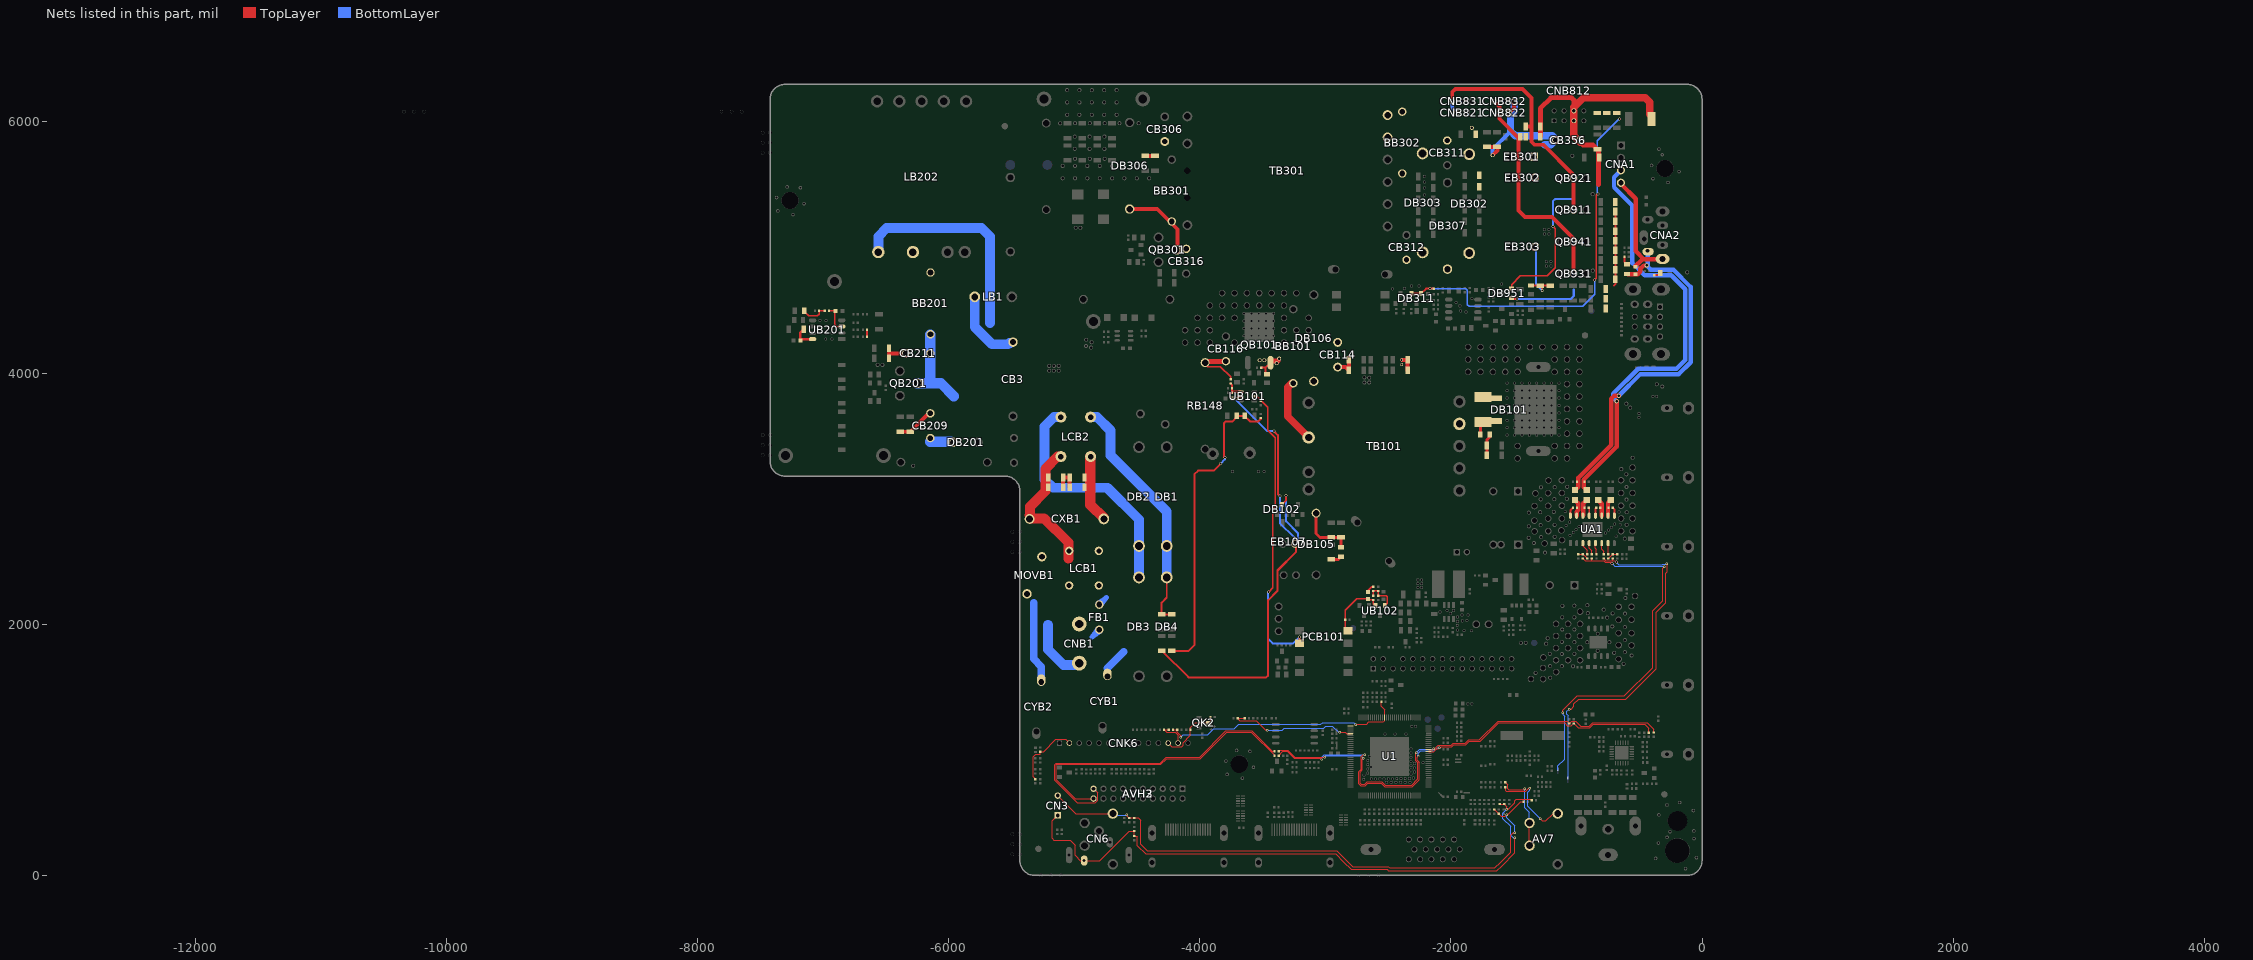
[diagram p0: the nets of this part, all layers, seen from the top]
# Altium PCB MISC84277.PcbDoc (part 11 of 15)
Units mil, origin at the board's own origin, x right, y up, seen from the top; angles counter-clockwise.
Board outline 7422.08 x 6299.21 mil, 2 copper layers (TopLayer, BottomLayer), stack 61.855 mil thick; 709 components, 395 nets, 2812 pads, 811 vias.

## Via types
v1: diameter 23.62, hole 15.75, TopLayer to BottomLayer, tented both sides, 437 vias
v2: diameter 19.68, hole 11.81, TopLayer to BottomLayer, tented both sides, 353 vias
v3: diameter 31.5, hole 23.62, TopLayer to BottomLayer, tented both sides, 16 vias
v4: diameter 31.5, hole 19.68, TopLayer to BottomLayer, tented both sides, 4 vias
v5: diameter 17.72, hole 9.84, TopLayer to BottomLayer, tented both sides, 1 vias

## Nets (pads, with @x,y where several pads share a name; then routed paths per layer and width w, separated by ;. In a path a pad name is that pad's centre, name@x,y a point inside that pad or via, vN(x,y) a via of type N, cw(c..) or ccw(c..) an arc to the next point about the centre after c; other vN are vias at no path point) (continued)
K7: CNK6.2 RK5.2 RK6.2 | length 552.8
  TopLayer w5: RK6.2@-5308.96,769.93 -5312.43,769.93 -5327.79,785.29 -5327.79,943.38 -5308.61,962.56 -5274.6,962.56 -5271.45,965.71 RK5.2@-5271.45,984.62 -5244.79,984.62 -5146.96,1082.45 -5068.22,1082.45 CNK6.2@-5039.07,1053.3
KEY: CK2.1 RK3.1 U1.101 | length 1020.6
  TopLayer w6: RK3.1@-3642.73,1251 CK2.1@-3698.27,1250.99 -3680.43,1233.16 -3551.66,1233.16 -3475.5,1157 v2@-3464.3,1157 ; v2@-2883,1139 -2842.97,1139 -2831.75,1127.78 U1.101@-2800.46,1127.78
  BottomLayer w6: v2@-3464.3,1157 -3344.2,1157 -3328.78,1172.42 -3012.14,1172.42 -2995.56,1189 -2944.68,1189 v2@-2893.68,1138
  other v2: -2884,1138 -3462.8,1156.4
L: DB1.A DB4.K LCB2.3 RB101.1 RB141.2 | length 1949.2
  TopLayer w15.75: DB4.K@-4263.49,2373.12 -4263.49,2213.01 -4304.29,2172.21 RB101.1@-4304.29,2078.76 RB141.2@-4224.49,2078.76
  BottomLayer w78.74: LCB2.3@-4869.89,3650.02 -4818.62,3650.02 -4710,3541.4 -4710,3344.3 -4263.49,2897.79 DB4.K@-4263.49,2373.12
L-1: CNB1.1 FB1.1
L-2: FB1.2 LCB1.2@-4804.49,2308.7
L-3: CXB1.1 CYB1.2 LCB1.3@-4804.49,2584.3 LCB2.2 MOVB1.2@-5258.54,2537.24 RB1.1 RB2.1 | length 723.5
  TopLayer w82.68: LCB2.2@-4869.89,3335.06 -4872.2,3332.74 -4872.2,2952.78 CXB1.1@-4762.92,2843.5
  BottomLayer w59.06: -4735.81,1650.69 -4604.51,1781.99
L-N: RB1.2 RB2.2 RB3.1 RB4.1 | length 209
  TopLayer w31.5: RB4.1@-5089.33,3090.94 RB3.1@-5089.33,3169.17 RB1.2@-5036.74,3169.17 RB2.2@-5036.74,3090.94
LED1: CNB821.2 CNB831.3 DB951.3 QB911.C QB921.C RB905.1 | length 3165.6
  TopLayer w11.81: DB951.3@-1517.68,4674.29 -1517.68,4705.32 -1447.41,4775.59 -1234.25,4775.59 -1171.26,4838.58 -1171.26,5150.26 v1(-1189,5168)
  TopLayer w31.5: CNB831.3@-1989.88,6163.14 -1989.88,6237.58 -1964.5,6262.96 -1431.77,6262.96 -1358.2,6189.4 -1358.2,5968.4 ; RB905.1@-1392,5963.8 -1362.8,5963.8 -1358.2,5968.4 ; QB911.C@-1022.5,5307.26 -1022.5,5578 -1263,5818.5 -1334.2,5818.5 -1358.2,5842.5 -1358.2,5968.4
  BottomLayer w15.75: v1(-1189,5168) -1189,5367.5 -1170,5386.5 -1039.5,5386.5 -1022.5,5369.5 QB911.C@-1022.5,5307.26
  BottomLayer w31.5: CNB831.3@-1989.88,6163.14 -1989.88,6111.52 CNB821.2@-1950.51,6072.15
LED2: CNB822.2 CNB832.3 DB951.1 JB102.2 JB107.1 pad.VIA5@-1833.15,5953.3 QB931.C QB941.C RB904.1 | length 2353.7
  TopLayer w19.68: DB951.1@-1517.68,4599.29 -1508.89,4590.5 v1(-1475,4590.5)
  TopLayer w31.5: CNB832.3@-1654.61,6163.14 -1615.24,6123.77 CNB822.2@-1615.24,6072.15 -1615.24,6026.66 -1469.78,5881.2 -1445.6,5881.2 -1460.63,5866.17 -1460.63,5295.28 -1409.45,5244.09 -1194.96,5244.09 -1022.5,5071.63 QB931.C@-1022.5,4792.7
  BottomLayer w19.68: v1@-1475,4590.13 -1350,4590.13 ; -1362,4590.13 -1350,4590.13 ; -1022.5,4662.5 -1022.5,4614 -1046.37,4590.13 -1350,4590.13
LED+: CB312.2 CB356.2 CNB822.1 CNB832.1 DB302.K DB303.K DB307.A EB301.1 EB302.1 EB303.1 JB103.1 JB106.1 pad.VIA5@-1668.9,5735.1 RB358.1 RB360.2 RB363.2 | length 1818.8
  TopLayer w15.75: RB358.1@-1363,4697.59 RB363.2@-1210.69,4697.59 ; RB360.2@-1288.48,4696.65 -1274.94,4696.65 -1273,4694.71 v1(-1273,4658)
  TopLayer w31.5: JB103.1@-1714.4,5801.14 -1714,5801.54 JB106.1@-1632.9,5801.54 ; pad.VIA5@-1668.9,5735.1 -1630.5,5773.5 -1630.5,5800.44 JB106.1@-1616.88,5800.44 ; CNB822.1@-1536.5,6072.15 -1497.13,6111.52 CNB832.1@-1497.13,6163.14
  BottomLayer w15.75: EB303.1@-1322.83,4988.76 -1322.83,4707.83 v1(-1273,4658)
  BottomLayer w31.5: pad.VIA5@-1669.2,5735.1 -1669.2,5782.9 -1539.5,5912.6 ; -1298.2,5889.5 -1297.2,5890.5
  BottomLayer w59.06: CNB832.1@-1497.13,6163.14 -1497.13,6085.87 -1526,6057 -1526,5927.7 -1487.8,5889.5 -1298.2,5889.5 -1192.43,5889.5 -1163.28,5860.35 CB356.2@-1167.43,5856.2 -1205.63,5818 -1253.36,5818
LED_FB: CB356.1 CNB812.5 CNB812.6 DB310.A DB311.1 DB311.3 RB337.2 RB338.2 RB339.2 RB340.2 RB341.2 RB351.1 RB904.2 RB905.2 RB911.1 RB912.1 RB913.1 RB921.1 RB922.1 RB923.1 RB931.1 RB932.1 RB933.1 RB941.1 RB942.1 RB943.1 | length 5802.8
  TopLayer w11.81: v1(-856.3,4740.15) -842.39,4754.05 -842.39,5415.21 v1(-830.7,5426.9)
  TopLayer w15.75: DB311.3@-2312.5,4634.5 DB311.1@-2237.5,4634.5 -2198.57,4673.43 v1@-2168.5,4673.43 ; v1@-2165.5,4673.43 RB351.1@-2137.3,4673.43 ; -702.13,4696.87 -690.23,4708.77 RB922.1@-690.23,5274
  TopLayer w39.37: RB904.2@-1287.5,5888.74 -1287.5,6108.49 -1202.49,6193.5 -1041.02,6193.5 -1020.8,6173.28 -1020.8,6117.2 CNB812.6@-1020.8,6088.35 ; CB356.1@-970.07,5838.83 -949.25,5818 -870.5,5818 -824.5,5772 -824.5,5502.9
  TopLayer w59.06: CNB812.6@-1020.8,6088.35 CNB812.5@-1020.8,6009.61 -1020.8,5889.55 CB356.1@-970.07,5838.83 ; -1020.8,6117.2 -944.5,6193.5 -453.3,6193.5 -418,6158.2 DB310.A@-418,6061.2
  BottomLayer w11.81: v1(-2168.5,4672) -1883,4672 -1869,4658 -1869,4545.63 -1856,4532.63 -950.16,4532.63 -856.3,4626.49 v1(-856.3,4740.15) ; v1(-830.7,5426.9) -834.65,5430.85 -834.65,5849.75 v1(-659,6025.4)
LED_G: CK3.2 CNK6.12 QK2.C RK2.1 | length 504.6
  TopLayer w5: CNK6.12@-4251.67,1053.3 -4222.07,1023.7 -4143.8,1023.7 -4132.9,1034.6 -4132.9,1055.82 -4074.87,1113.85 CK3.2@-4074.87,1160.01 CK3.2@-4074.87,1160.6 ; CK3.2@-4075.16,1160.3 CK3.2@-4074.87,1160.6 ; QK2.C@-3940.33,1213.8 -4036.04,1213.8 -4074.87,1174.97 CK3.2@-4074.87,1160.6 ; QK2.C@-3929.37,1213.8 -3914.23,1228.94 RK2.1@-3914.23,1261.1
LED_R: CK10.2 CNK6.13 RK21.2 | length 229.8
  TopLayer w6: RK21.2@-4247.33,1160 -4284.46,1160 -4263.86,1139.4 -4195.9,1139.4 -4172.93,1116.43 CNK6.13@-4172.93,1053.3
LED_RED: RK18.1 RK20.2 RK21.1 U1.83 | length 1989.4
  TopLayer w6: RK21.1@-4213.87,1160 RK20.2@-4179.33,1160 -4179.33,1138.39 -4152.1,1111.16 v2(-4152.1,1100.4) ; v2(-2759,1200) -2756.5,1202.5 -2671.94,1202.5 -2652.94,1221.5 -2537.5,1221.5 -2528.81,1230.19 U1.83@-2528.81,1257.7 -2528.81,1320.37 -2553.73,1345.29 RK18.1@-2553.73,1381
  BottomLayer w6: v2(-4152.1,1100.4) -4131.83,1120.67 -4033.4,1120.67 ; -4062.3,1120.67 -4033.4,1120.67 ; v2@-2761,1198 v2(-2759,1200) -2776,1217 -3022.8,1217 -3037.8,1202 -3691.04,1202 -3725.69,1167.36 -3888.63,1167.36 -3935.32,1120.67 -4033.4,1120.67
LINEOUT-L: CN3.3 CN6.3 CO4.1 CO10.2 R2.2 RO7.2 RO15.2 | length 4702.3
  TopLayer w6: CN3.3@-5131.53,624.33 CN3.3@-5131.53,635.1 -4988.41,491.97 CN6.3@-4688.98,491.97 ; -2852.12,141.88 -2780.29,70.06 -2499.27,70.06 -2488.59,59.38 -1649.74,59.38 -1604.62,104.5
  TopLayer w8: v2(-4581.5,483.9) -4581.5,474.88 RO7.2@-4563.06,456.43 ; RO7.2@-4563.06,457.03 -4488.93,457.03 -4470.5,438.6 -4470.5,409.5 ; -4470.5,433.5 -4470.5,409.5 ; -2852.12,141.88 -2907.73,197.5 -4420.45,197.5 -4470.5,247.55 -4470.5,409.5 ; RO15.2@-1655,523.73 -1651.46,523.73 CO4.1@-1618,490.27 -1618,489 -1599,470 -1567,470 -1559.32,477.68 -1559.32,479.68 -1555.32,479.68 v2(-1555.32,483.07) -1547.05,483.07 -1445.85,584.27 -1422.73,584.27 R2.2@-1422.73,587 ; -1604.62,104.5 -1524.69,184.43 -1524.69,320.39 -1504.08,341 v2(-1491,341)
  BottomLayer w8: CN6.3@-4688.98,491.97 -4676.76,479.76 v2@-4585.64,479.76 ; v2(-1555.32,483.07) -1555.32,457.7 -1491,393.38 v2(-1491,341)
LINEOUT-R: CN3.1 CN6.2 CO1.1 CO11.2 R1.2 RO3.2 RO17.2 | length 5122.5
  TopLayer w6: -2855.91,108.91 -2795.06,48.06 -2508.38,48.06 -2497.7,37.38 -1634.11,37.38 -1592.98,78.5
  TopLayer w8: CN3.1@-5131.53,477.62 -5175.4,433.75 -5175.4,293.8 -5162.8,281.2 -5032,281.2 -4992.3,241.5 -4992.3,159.8 -4950.46,117.96 CN6.2@-4921.26,117.96 -4795.54,117.96 -4560.73,352.77 RO3.2@-4522.89,352.77 CO11.2@-4522.9,312.63 -4503.03,312.63 -4496.8,306.4 -4496.8,237.08 -4431.22,171.5 -2918.5,171.5 -2855.91,108.91 ; RO17.2@-1610,567.27 CO1.1@-1574,567.27 -1574,566 -1555,547 v2(-1555,527) -1544,527 -1492.16,578.84 -1492.16,595.68 -1481,606.84 -1366.57,606.84 R1.2@-1356.73,597 ; -1592.98,78.5 -1490.88,180.61 -1490.88,245 ; v2(-1491,300) -1491,245.12 -1490.88,245 ; -1490.88,271.52 -1490.88,245
  BottomLayer w8: v2(-1555,527) -1556.42,527 -1587.16,496.26 -1587.16,452.77 -1524.69,390.3 -1524.69,320.69 -1504,300 v2(-1491,300)
LOUT+: CA25.1 CA41.2 CNA2.5 LBA1.2 pad.VIA5@-442.4,4857.1 pad.VIA5@-663.82,3818.81 RA10.1 | length 2996.5
  TopLayer w15: CNA2.5@-445.34,4962.3 -433.07,4974.57 CNA2.5@-423.51,4965
  TopLayer w35: LBA1.2@-1012,3068 -985,3095 -985,3166.57 -723.5,3428.07 -723.5,3795.5 -700.72,3818.28 pad.VIA5@-664.35,3818.28 ; CA41.2@-590.2,4788.02 -512.28,4788.02 -491.6,4808.7 -491.6,4831.3 -465.8,4857.1 pad.VIA5@-442.4,4857.1
  BottomLayer w30: CNA2.5@-433.07,4974.57 CNA2.5@-419.02,4960.51
  BottomLayer w35: pad.VIA5@-663.82,3818.81 -490.63,3992 -185.69,3992 -94.5,4083.19 -94.5,4086.19 ; CNA2.5@-446.37,4959.17 CNA2.5@-433.07,4972.47 ; pad.VIA5@-442.4,4857.1 -407.78,4822.48 -227.85,4822.48 -91.5,4686.13 -91.5,4086.19 ; pad.VIA5@-433.07,4854.1 CNA2.5@-433.07,4972.31
LOUT+': CNA1.4 CNA2.7 RA10.2 | length 965.6
  TopLayer w35: CNA1.4@-646.5,5500.7 CNA1.4@-646.5,5516.04 ; CNA1.4@-646.5,5505.5 -529,5388 -529,4972.3 -462.37,4905.67 ; RA10.2@-531.6,4851.2 -477.13,4905.67 -462.37,4905.67 ; CNA2.7@-314.96,4905.67 -462.37,4905.67
  BottomLayer w30: CNA2.7@-314.96,4905.67 CNA2.7@-280.03,4905.67
LOUT-: CA16.2 CNA1.3 LBA2.2 pad.VIA5@-680.5,3775.28 | length 3462.1
  TopLayer w35: LBA2.2@-920,3068 -944,3092 -944,3151 -680.5,3414.5 pad.VIA5@-680.5,3775.28
  BottomLayer w35: -701.5,5484.3 -701.5,5560.25 CNA1.3@-646.5,5615.25 ; -696,5474.1 -554.68,5332.78 -554.68,4876.08 -458.18,4779.58 -245.76,4779.58 -134.5,4668.32 -134.5,4104 -203.5,4035 -508.44,4035 -706.82,3836.62 -706.82,3800.63 pad.VIA5@-681.47,3775.28
M_SCL: RH19.1 RT3.2 RT6.1 U1.52 | length 3814.1
  TopLayer w5: RH19.1@-3371.57,989.2 -3363.67,997.1 -3298,997.1 ; -3325.3,997.1 -3298,997.1 ; -3020.84,941.94 -3056,941.94 ; v2@-3005.44,941.94 -3056,941.94 ; -1043,1223.8 -1039.6,1227.2 -1007.7,1227.2 -1002.2,1221.7 ; -3298,997.1 -3242.84,941.94 -3056,941.94
  TopLayer w6: v2@-2697.7,933.8 -2704.84,926.66 -2704.84,839.63 -2723.5,820.97 -2723.5,734.96 -2714.54,726 -2688.11,726 -2668.3,745.81 -2552.5,745.81 -2524.51,717.83 -2313.57,717.83 -2263.5,767.89 -2263.5,895.3 -2281.3,913.1 -2281.3,967.2 ; U1.52@-2178.42,1001.79 -2146.61,1001.79 ; v2@-2134.11,1004.62 -2102.73,1036 -1999.56,1036 -1983.06,1052.5 -1885.3,1052.5 -1859.3,1078.5 -1772.82,1078.5 -1624.27,1227.06 -1073.49,1227.06 RT3.2@-1057.92,1211.49 ; RT3.2@-1057.8,1211.37 -1055.43,1211.37 -1043,1223.8 ; -1002.2,1221.7 -966.7,1186.2 -899.1,1186.2 -870.04,1215.26 -438.36,1215.26 -385.62,1162.52 RT6.1@-385.62,1137.14
  TopLayer w7: RT6.1@-385.62,1137.14 RT6.1@-385.62,1140.02
  BottomLayer w5: v2(-3004.5,941) -3005.3,941.8 -2996,951.1 -2967,951.1
  BottomLayer w6: -2967,951.1 -2719.74,951.1 v2@-2696.85,928.21 ; v2(-2277,976.8) -2248.11,1005.69 -2142.72,1005.69 v2(-2138.95,1009.46)
  other v2: -2697.7,933.2
M_SCL_HDMI: AVH2.19 AVH3.19 RH19.2 | length 2580.1
  TopLayer w5: AVH2.19@-4846.48,689.7 -4813.98,657.2 -4813.98,597.5 -4833.01,578.46 -4975.1,578.46 -5155,758.36 -5155,880.74 -5142.15,893.59 -4314.35,893.59 -4268.24,939.7 -4002.65,939.7 -3791.69,1150.66 -3585.83,1150.66 -3424.37,989.2 RH19.2@-3405.03,989.2
M_SDA: RH20.1 RT4.2 RT5.1 U1.51 | length 3852.1
  TopLayer w5: RH20.1@-3371.57,953.5 RH20.1@-3371.57,954 -3338.47,987.1 -3302.14,987.1 -3246.98,931.94 -3037.74,931.94 v2(-3028.6,922.8)
  TopLayer w6: -2720.2,715 -2734.5,729.3 -2734.5,825.53 -2715.84,844.19 -2715.84,944.16 v2@-2697.9,962.1 ; -2719.1,715 -2683.56,715 -2663.81,734.74 -2650.9,734.74 ; -2650.9,734.81 -2557.05,734.81 -2529.07,706.83 -2309.01,706.83 -2252.5,763.34 -2252.5,899.85 -2270.3,917.65 -2270.3,941.24 v2(-2261.03,950.51) ; U1.51@-2178.42,986.05 -2137.13,986.05 -2112.88,1010.29 v2@-2100.11,1010.29 ; v2@-2089.81,1013.68 -2078.49,1025 -1995,1025 -1978.5,1041.5 -1880.74,1041.5 -1854.74,1067.5 -1768.27,1067.5 -1619.71,1216.06 -1095.46,1216.06 -1072.5,1193.1 -1040.6,1193.1 RT4.2@-1029.44,1204.26 ; RT4.2@-1021.7,1210.37 -986.53,1175.2 -894.54,1175.2 -865.48,1204.26 -457.1,1204.26 -422.97,1170.13 RT5.1@-422.97,1136.59
  BottomLayer w5: v2(-3028.6,922.8) -3028.6,942.17 -3008.67,962.1
  BottomLayer w6: -3008.67,962.1 v2(-2688.2,962.1) ; v2@-2259.16,952.38 -2259.16,974.04 -2241.59,991.61 -2131.49,991.61 -2106.8,1016.3 v2@-2094.11,1016.3
  other v2: -2093.27,1017.13
M_SDA_HDMI: AVH2.20 AVH3.20 RH20.2 | length 2403.6
  TopLayer w5: AVH2.20@-4846.48,610.96 -4993.46,610.96 -5145,762.5 -5145,876.6 -5138.01,883.59 -4310.2,883.59 -4264.09,929.7 -3998.51,929.7 -3787.55,1140.66 -3589.97,1140.66 -3405.03,955.72 RH20.2@-3405.03,953.5
MHL_DET: U1.97
N-1: CNB1.3 LCB1.1 | length 499.2
  BottomLayer w78.74: -5210.5,1995.5 -5210.5,1799.5 -5085.2,1674.2 CNB1.3@-4959.2,1674.2
N-2: CXB1.2 CYB2.2 LCB1.4@-5040.71,2584.3 LCB2.1@-5106.11,3335.06 MOVB1.1 RB3.2 RB4.2 | length 1879.4
  TopLayer w78.74: -5229,3147.61 -5229,3090.94 ; LCB2.1@-5106.11,3335.06 -5132.14,3335.06 -5229,3238.2 -5229,3090.94 ; -5047.11,2521.8 -5047.11,2650.61 -5240,2843.5 CXB1.2@-5333.72,2843.5 ; CXB1.2@-5353.48,2863.25 CXB1.2@-5333.72,2843.5 ; CXB1.2@-5353.48,2863.25 CXB1.2@-5353.48,2872.85 ; CXB1.2@-5353.48,2863.25 -5353.48,2843.5 CXB1.2@-5333.72,2843.5 ; CXB1.2@-5353.48,2863.25 -5358.28,2868.06 CXB1.2@-5353.48,2872.85 ; CXB1.2@-5353.48,2872.85 -5353.48,2936.08 -5229,3060.56 -5229,3090.94
  BottomLayer w59.06: -5323.5,2171.74 -5323.5,1724 -5262.01,1662.51 CYB2.2@-5262.01,1540.35
N-3: DB2.A DB3.K LCB2.4 | length 1927.2
  BottomLayer w78.74: LCB2.4@-5106.11,3650.02 -5160.04,3650.02 -5236.22,3573.83 -5236.22,3153.28 -5169.5,3086.56 -4736.87,3086.56 -4484.49,2834.17 DB3.K@-4484.49,2373.12
NetAV7_3: AV7.3 RV6.2 | length 707.3
  TopLayer w7: RV6.2@-1565.27,701.01 -1565.27,675.27 -1559.34,669.34 -1405.66,669.34 -1381,694 v2(-1371,694)
  TopLayer w8: v2(-1289.24,452.24) -1272,435 -1244,435 -1186.87,492.13 -1145.67,492.13 -1145.67,483 AV7.3@-1146.67,482
  BottomLayer w8: v2(-1371,694) -1371,677.62 -1388,660.62 -1388,551 v2(-1289.24,452.24)
NetAV7_4: AV7.4 AV7.5@-1374.02,417.32 RV7.2 | length 666
  TopLayer w7: RV7.2@-1565.27,737.27 -1548,720 -1548,690 -1539.34,681.34 -1421.66,681.34 v2@-1415.16,687.84 ; RV7.2@-1565.27,740 RV7.2@-1564.27,739
  TopLayer w8: RV7.2@-1565.27,737.27 RV7.2@-1565.27,739 ; v2@-1415.16,687.84 v2(-1414,689) ; AV7.4@-1377.95,236.22 AV7.5@-1377.95,417.32
  BottomLayer w8: v2(-1414,689) -1414,538.27 -1377.95,502.22 AV7.5@-1377.95,417.32
NetBB101_2: BB101.2 TB101.3@-3133.09,3487.4 | length 532.2
  TopLayer w59.06: BB101.2@-3269,3918.72 -3300.25,3887.48 -3300.25,3654.55 TB101.3@-3133.09,3487.4 TB101.3@-3151.83,3487.4
NetBB201_1: BB201.1 LB202.3@-6284.9,4963.91
NetBB201_2: BB201.2 CB209.2 CB211.1 DB201.A QB201.D@-6251.52,3917.89 | length 876.1
  BottomLayer w82.68: QB201.D@-6251.52,3917.89 -6061.39,3917.89 -5960.5,3817 ; -6146.57,3927.32 CB211.1@-6146.57,4157 BB201.2@-6146.57,4307.3 ; CB209.2@-6146,3453.07 DB201.A@-5982.64,3453.07
NetBB301_1: BB301.1 CB316.2 DB306.A QB301.D@-4190.51,4982.37 | length 592
  TopLayer w31.5: DB306.A@-4525.08,5307.83 -4339.33,5307.83 -4177,5145.5 QB301.D@-4177,4968.86
NetBB302_1: BB302.1 TB301.5@-2504.74,5877.25 TB301.6
NetBB302_2: BB302.2 CB311.1 DB302.A DB303.A RB328.1 RB332.1
NetCA12_1: CA12.1 UA1.13 | length 64.6
  TopLayer w15: CA12.1@-903.27,2927 -899.02,2922.75 UA1.13@-899.02,2864.19
NetCA12_2: CA12.2 LBA2.1 UA1.14 | length 131.6
  TopLayer w35: UA1.14@-946,2867.21 -946,2962 LBA2.1@-920,2988
NetCA13_1: CA13.1 UA1.12 | length 65
  TopLayer w15: UA1.12@-849.02,2864.19 -849.02,2921.73 CA13.1@-843.73,2927.02
NetCA13_2: CA13.2 LBA3.1 UA1.11 | length 141.4
  TopLayer w35: LBA3.1@-827,2988 -799.02,2960.02 -799.02,2927.01 ; UA1.11@-799.02,2864.19 -799.02,2927.01 ; -799.02,2933.02 -799.02,2927.01
NetCA14_1: CA14.1 UA1.16 | length 88.6
  TopLayer w15: UA1.16@-1049.02,2864.19 -1049.02,2906.73 CA14.1@-1028.73,2927.02 -1041.02,2914.73
NetCA14_2: CA14.2 LBA1.1 UA1.15 | length 140
  TopLayer w35: LBA1.1@-1012,2988 -986,2962 -986,2910 -999.02,2896.98 UA1.15@-999.02,2864.19
NetCA15_2: CA15.2 UA1.5 | length 91.8
  TopLayer w8: UA1.5@-849.02,2645.69 -849.02,2603.52 -840.99,2595.49 CA15.2@-840.99,2557.23
NetCA18_1: CA18.1 UA1.3 | length 92.3
  TopLayer w8: UA1.3@-957.02,2631.52 -913.47,2587.97 CA18.1@-913.47,2557.23
NetCA18_2: CA18.2 CA31.2 RA4.2 | length 86.5
  TopLayer w8: RA4.2@-986,2557.23 CA31.2@-949.74,2557.23 -946.73,2557.23 -913.48,2523.98 CA18.2@-913.48,2523.77
NetCA19_1: CA19.1 UA1.4 | length 97.5
  TopLayer w8: UA1.4@-899.02,2645.69 -899.02,2605.79 -877.22,2584 CA19.1@-877.22,2557.23
NetCA19_2: CA19.2 CA31.1 RA7.JP_1K | length 2888.4
  TopLayer w8: v2(-1109,1294) -1109,1313.65 -993.8,1428.84 -620.47,1428.84 -394.74,1654.57 -394.74,2106.5 -315,2186.24 -315,2444 v2(-300,2459) ; CA31.1@-949.74,2523.77 -931.88,2505.91 -879.34,2505.91 ; CA19.2@-877.23,2523.77 -879.34,2521.65 -879.34,2505.91 ; v1@-717.5,2492.91 -771.25,2492.91 -784.25,2505.91 -879.34,2505.91
  BottomLayer w8: RA7.JP_1K@-1148.31,844.05 -1148.31,872.69 -1094.84,926.16 -1094.84,1266.07 -1107,1278.23 -1107,1292 v2(-1109,1294) ; v1(-717.5,2484) -694.02,2460.52 -301.52,2460.52 v2(-300,2459)
NetCA20_1: CA20.1 UA1.7 | length 89.1
  TopLayer w8: UA1.7@-749.02,2645.69 -747.47,2644.15 CA20.1@-747.47,2557.23
NetCA20_2: CA20.2 CA32.1 RA12.2 | length 86.3
  TopLayer w8: CA20.2@-747.48,2523.77 -744.69,2523.77 CA32.1@-711.22,2557.23 RA12.2@-675,2557.23
NetCA21_1: CA21.1 UA1.6 | length 98
  TopLayer w8: UA1.6@-796.72,2643.4 UA1.6@-799.02,2645.69 -799.02,2595.52 -783.72,2580.22 CA21.1@-783.72,2557.23
NetCA21_2: CA21.2 CA32.2 RA11.JP_1K | length 2811.6
  TopLayer w8: v2(-1059,1324) -1044,1324 -1021,1347 -1021,1364.88 -983.04,1402.84 -609.7,1402.84 -366.74,1645.8 -366.74,2094.9 -289,2172.64 -289,2406 -277.16,2417.84 -277.16,2480.16 v2(-280,2483) ; CA21.2@-783.73,2523.77 -765.87,2505.91 -694.91,2505.91 v1(-683.5,2494.5) ; -711.23,2507.63 CA32.2@-711.23,2523.77
  BottomLayer w8: RA11.JP_1K@-1066.84,780 -1066.84,1274.84 -1076.84,1284.84 -1076.84,1305.16 -1059,1323 v2(-1059,1324) ; v1(-683.5,2494.5) -662.52,2473.52 -318.48,2473.52 -313,2479 -284,2479 v2(-280,2483)
NetCA22_1: CA22.1 UA1.9 | length 67.9
  TopLayer w15: CA22.1@-711.27,2927 -699.02,2914.75 UA1.9@-699.02,2864.19
NetCA22_2: CA22.2 LBA4.1 UA1.10 | length 132.5
  TopLayer w35: UA1.10@-749.02,2864.19 -749.02,2966.98 LBA4.1@-728,2988
NetCA40_1: CA40.1 RA23.2 | length 60.9
  TopLayer w15: RA23.2@-376.16,4781.79 -338.91,4781.79 CA40.1@-322.19,4798.5
NetCA41_1: CA41.1 RA28.2 | length 67.2
  TopLayer w15: RA28.2@-616.95,4924.87 -616.95,4884.08 CA41.1@-598.3,4865.43
NetCB3_1: CB3.1 LB1.2 LB202.1 | length 2383.1
  BottomLayer w78.74: LB202.1@-6560.49,4963.91 -6560.49,5089.12 -6494.09,5155.51 -5891.72,5155.51 ; -5848.11,5155.51 -5891.72,5155.51 ; LB1.2@-5792.64,4607.5 -5792.64,4367.44 -5654.7,4229.5 -5526.28,4229.5 CB3.1@-5514.7,4241.08 ; -5671.26,4397.64 -5671.26,5086.76 -5740.01,5155.51 -5891.72,5155.51
NetCB101_1: CB101.1 RB103.2 RB105.1 UB101.4 | length 153.6
  TopLayer w15.75: RB105.1@-3755,3916.77 -3742.77,3904.54 RB103.2@-3742.77,3843 -3733.87,3851.9 UB101.4@-3671.65,3851.9
NetCB102_1: CB102.1 DB102.2 EB107.1 RB102.2 UB101.5 | length 4042.6
  TopLayer w15.75: RB102.2@-4304.29,1788.35 -4302.13,1788.35 -4089.85,1576.07 ; -4092.52,1578.74 -4089.85,1576.07 ; CB102.1@-3740.69,3798 v1@-3707.45,3798 ; v1(-3706.69,3797.24) v1@-3707.45,3798 ; UB101.5@-3671.65,3814.5 -3690.95,3814.5 v1@-3707.45,3798 ; v1(-3409.45,3537.4) -3377.72,3505.67 -3377.72,3037.17 v1(-3362.2,3021.65) ; DB102.2@-3347,2953.53 -3312.99,2987.54 v1(-3312.99,3023.62) ; EB107.1@-3233.79,2640.07 -3233.79,2575.71 -3381.5,2428 -3381.5,2266.14 -3456.07,2191.57 -3456.07,1591.82 -3471.7,1576.18 -3533.74,1576.18 -3533.86,1576.07 -4089.85,1576.07
  BottomLayer w15.75: v1(-3706.69,3797.24) -3706.69,3781.49 -3462.6,3537.4 v1(-3409.45,3537.4) ; v1(-3362.2,3021.65) -3362.2,2805.12 -3248.07,2690.99 EB107.1@-3248.07,2654.36 ; v1(-3312.99,3023.62) -3312.99,2818.9 -3216.54,2722.44 -3216.54,2657.32 EB107.1@-3233.79,2640.07
NetCB103_1: CB103.1 PCB101.4 UB101.2 | length 2376.5
  TopLayer w11.81: UB101.2@-3565.35,3814.5 -3545.87,3814.5 -3460.51,3729.14 -3460.51,3545.59 -3399.5,3484.58 -3399.5,2939.08 -3419.29,2919.29 -3419.29,2289.21 v1(-3452,2256.5) ; CB103.1@-3513,3776.73 CB103.1@-3513,3781.63
  TopLayer w15.75: PCB101.4@-3205.13,1849.5 v1(-3205.13,1898.87)
  BottomLayer w15.75: v1(-3452,2256.5) -3456.07,2252.43 -3456.07,1882.5 -3421.07,1847.5 -3256.5,1847.5 v1(-3205.13,1898.87)
NetCB109_1: CB109.1 CB110.1 PCB101.2 RB132.2 UB102.K | length 516.4
  TopLayer w11.81: PCB101.2@-2800.2,1970.18 PCB101.2@-2820.87,1949.5 -2841.54,1970.16 RB132.2@-2841.54,2037.4 -2841.54,2111.22 -2750.25,2202.5 CB109.1@-2661.42,2202.5 -2652.81,2193.9 CB110.1@-2618.12,2193.9 -2618.12,2163.92 UB102.K@-2602.46,2148.27
NetCB109_2: CB109.2 RB133.1 | length 55.8
  TopLayer w11.81: CB109.2@-2661.42,2267.97 -2631.16,2298.23 RB133.1@-2618.11,2298.23
NetCB110_2: CB110.2 RB133.2 RB134.1 RB135.2 UB102.R | length 268.5
  TopLayer w11.81: CB110.2@-2618.12,2227.36 RB133.2@-2618.11,2264.76 RB134.1@-2580.71,2264.76 RB135.2@-2580.71,2228.22 ; RB135.2@-2580.71,2227.36 RB135.2@-2580.71,2228.22 ; UB102.R@-2527.46,2148.27 -2507.75,2167.98 -2507.75,2220.07 -2515.89,2228.22 RB135.2@-2580.71,2228.22
NetCB111_2: CB111.2 CB112.2 RB142.1 RB143.1 | length 2480.4
  TopLayer w15.75: RB142.1@-4224.49,1788.35 -4089.15,1788.35 -4044.31,1833.19 -4044.31,3193.06 -4013.37,3224 -3890.17,3224 v1(-3834.65,3279.53) ; v1@-3806.96,3332.55 -3806.96,3602.49 -3796.49,3612.96 -3743.34,3612.96 CB112.2@-3700.88,3655.42 ; CB112.2@-3696.3,3660 CB111.2@-3640.53,3660 -3640.53,3656.28 -3600.39,3616.14 -3533.46,3616.14 -3513,3636.61 RB143.1@-3513,3641.77
  BottomLayer w15.75: v1(-3834.65,3279.53) -3801.17,3313 v1(-3801.17,3326.76)
NetCB113_1: CB113.1 DB105.A RB114.1 RB115.1 | length 450.9
  TopLayer w23.62: DB105.A@-3074,2884.56 -3074,2722.5 -3042.94,2691.44 RB114.1@-2954.5,2691.44 RB115.1@-2875.97,2691.44 ; CB113.1@-2875.84,2613.35 RB115.1@-2875.84,2691.32
NetCB113_2: CB113.2 RB116.2 | length 87.3
  TopLayer w23.62: RB116.2@-2954.39,2516.27 -2896.86,2516.27 CB113.2@-2875.84,2537.29
NetCB114_1: CB114.1@-2902.49,4047.94 RB117.2 RB118.2 | length 183.5
  TopLayer w31.5: CB114.1@-2902.49,4047.94 -2839.39,4047.94 RB118.2@-2813.46,4022 RB117.2@-2813.46,4105.75
NetCB114_2: CB114.2 DB106.K pad.VIA5@-2392.66,4067.75 pad.VIA5@-2392.66,4105.75 RB145.2 RB147.2 | length 125.3
  TopLayer w31.5: pad.VIA5@-2386.75,4105.75 RB145.2@-2345.19,4105.75 RB147.2@-2345.19,4022
NetCB116_1: CB116.1 pad.VIA5@-3368.11,4116.14 pad.VIA5@-3387.8,4078.74 pad.VIA5@-3486.22,4102.36 pad.VIA5@-3524.22,4102.36 QB101.S RB105.2 RB108.2 RB109.2 RB148.2 | length 693.1
  TopLayer w11.81: RB148.2@-3952.48,4093.49 -3952.2,4093.21 -3952.2,4064.96 -3938.42,4051.18 -3887.8,4051.18 ; -3844.49,4051.18 -3887.8,4051.18 ; RB105.2@-3755,3950.23 -3755,3970.5 -3835.68,4051.18 -3887.8,4051.18
  TopLayer w15.75: RB109.2@-3510.82,4042.75 -3477.25,4042.75 ; RB108.2@-3477.25,4003.21 -3477.25,4042.75 ; QB101.S@-3437,4083 -3477.25,4042.75
  TopLayer w39.37: RB148.2@-3952.48,4093.49 -3790.41,4093.49 CB116.1@-3785.45,4088.53 ; QB101.S@-3437,4083 -3424.93,4095.07 -3376.57,4095.07
NetCB118_1: CB118.1 DB101.1 DB101.3 TB101.10 | length 88.5
  TopLayer w23.62: CB118.1@-1765.53,3511.5 DB101.3@-1765.53,3600
NetCB118_2: CB118.2 RB123.1 RB124.1 | length 176.7
  TopLayer w23.62: RB123.1@-1713.59,3344.78 -1713.59,3469.41 -1689.47,3493.53 CB118.2@-1689.47,3511.5
NetCB201_2: CB201.2 RB225.1 UB201.3 | length 217.1
  TopLayer w11.81: RB225.1@-6953.48,4496.35 -6908.21,4496.35 -6908.21,4388.59 -6889.99,4370.37 UB201.3@-6851.71,4370.37
NetCB206_2: CB206.2 RB210.1 UB201.8 | length 206.1
  TopLayer w19.68: RB210.1@-7154.88,4349.5 -7182.03,4322.35 CB206.2@-7182.03,4257.84 -7169.5,4270.37 UB201.8@-7084,4270.37
NetCB209_1: CB209.1 RB219.1 RB220.1 | length 296
  TopLayer w31.5: RB220.1@-6385.37,3532.99 RB219.1@-6305.64,3532.99 -6169.02,3669.61 CB209.1@-6146,3669.61
NetCB211_2: CB211.2 RB223.1 RB224.1 | length 132.9
  TopLayer w31.5: -6475.32,4154.5 -6472.81,4157 CB211.2@-6343.43,4157
NetCB212_1: CB212.1 RB225.2 RB227.2 | length 214
  TopLayer w11.81: CB212.1@-7148.72,4496.35 -7148.72,4488.72 -7116.21,4456.21 -7046.29,4456.21 -7032.22,4470.28 RB227.2@-7032.22,4496.35 -6989.47,4496.35 RB225.2@-6988.21,4497.61
NetCB221_2: CB221.2 RB221.1 | length 55.3
  TopLayer w15.75: CB221.2@-6649.66,4290.01 RB221.1@-6649.66,4345.31
NetCB306_1: CB306.1@-4279.5,5844.57 RB314.1 RB315.1 | length 78.7
  TopLayer w31.5: RB314.1@-4435.6,5729.4 RB315.1@-4356.88,5729.4